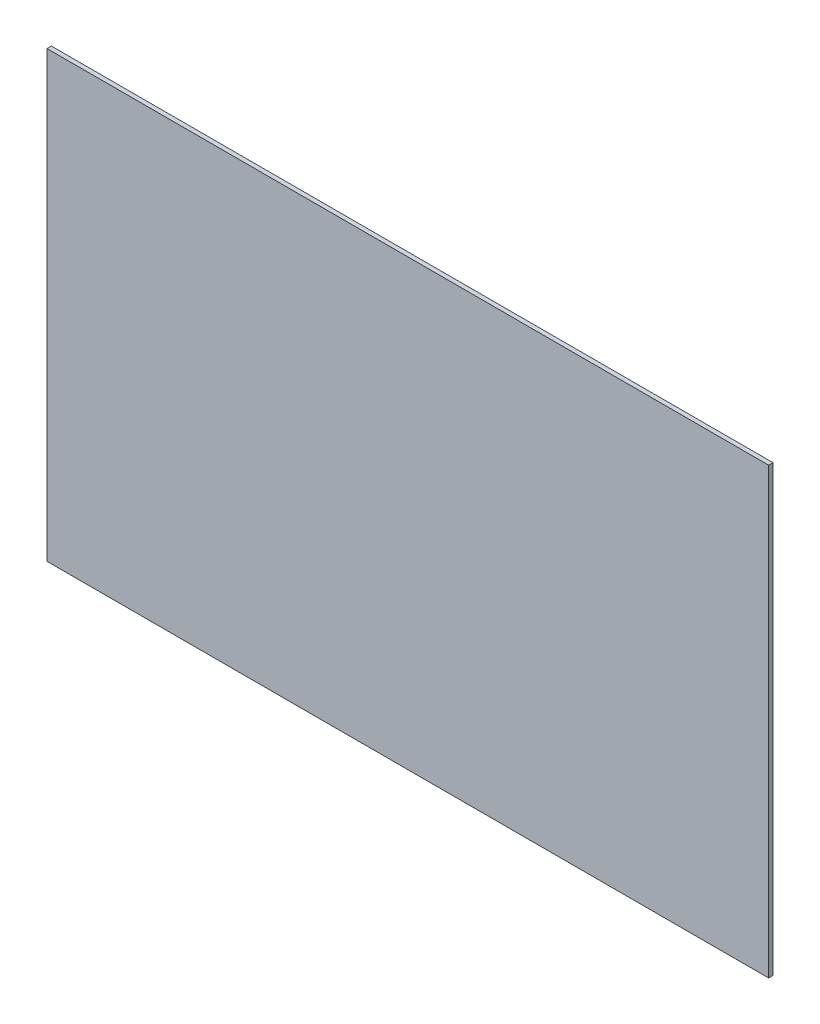
from build123d import *

# Parameters (mm, degrees)
SKETCH1_W           = 330.2
SKETCH1_H           = 203.2
BOSS_EXTRUDE1_DEPTH = 1


with BuildPart() as part:
    # Sketch1 → Boss-Extrude1 (new, symmetric)
    with BuildSketch(Plane.XY):
        Rectangle(SKETCH1_W, SKETCH1_H)
    extrude(amount=BOSS_EXTRUDE1_DEPTH, both=True)


solid = part.part
